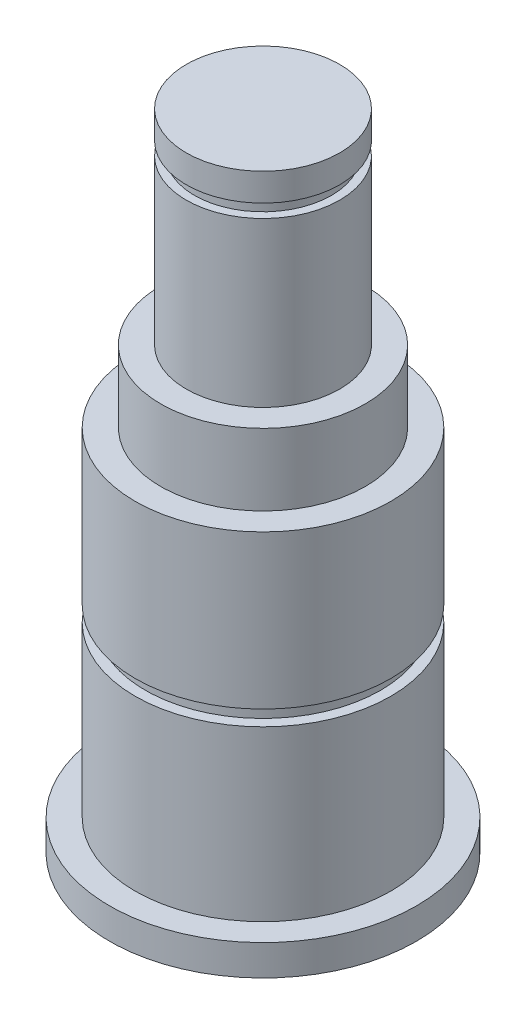
from build123d import *


with BuildPart() as part:
    # 草图1 → 旋转1 (revolve)
    with BuildSketch(Plane.XY):
        Polygon((7.5, 65.705286307), (0, 65.705286307), (0, 2.705286307), (15, 2.705286307), (15, 5.705286307), (12.5, 5.705286307), (12.5, 22.205286307), (11.5, 22.205286307), (11.5, 23.705286307), (12.5, 23.705286307), (12.5, 38.705286307), (10, 38.705286307), (10, 45.705286307), (7.5, 45.705286307), (7.5, 61.705286307), (6.7, 61.705286307), (6.7, 63.005286307), (7.5, 63.005286307), align=None)
    revolve(axis=Axis((0, 65.705286307, 0), (0, -1, 0)))


solid = part.part
